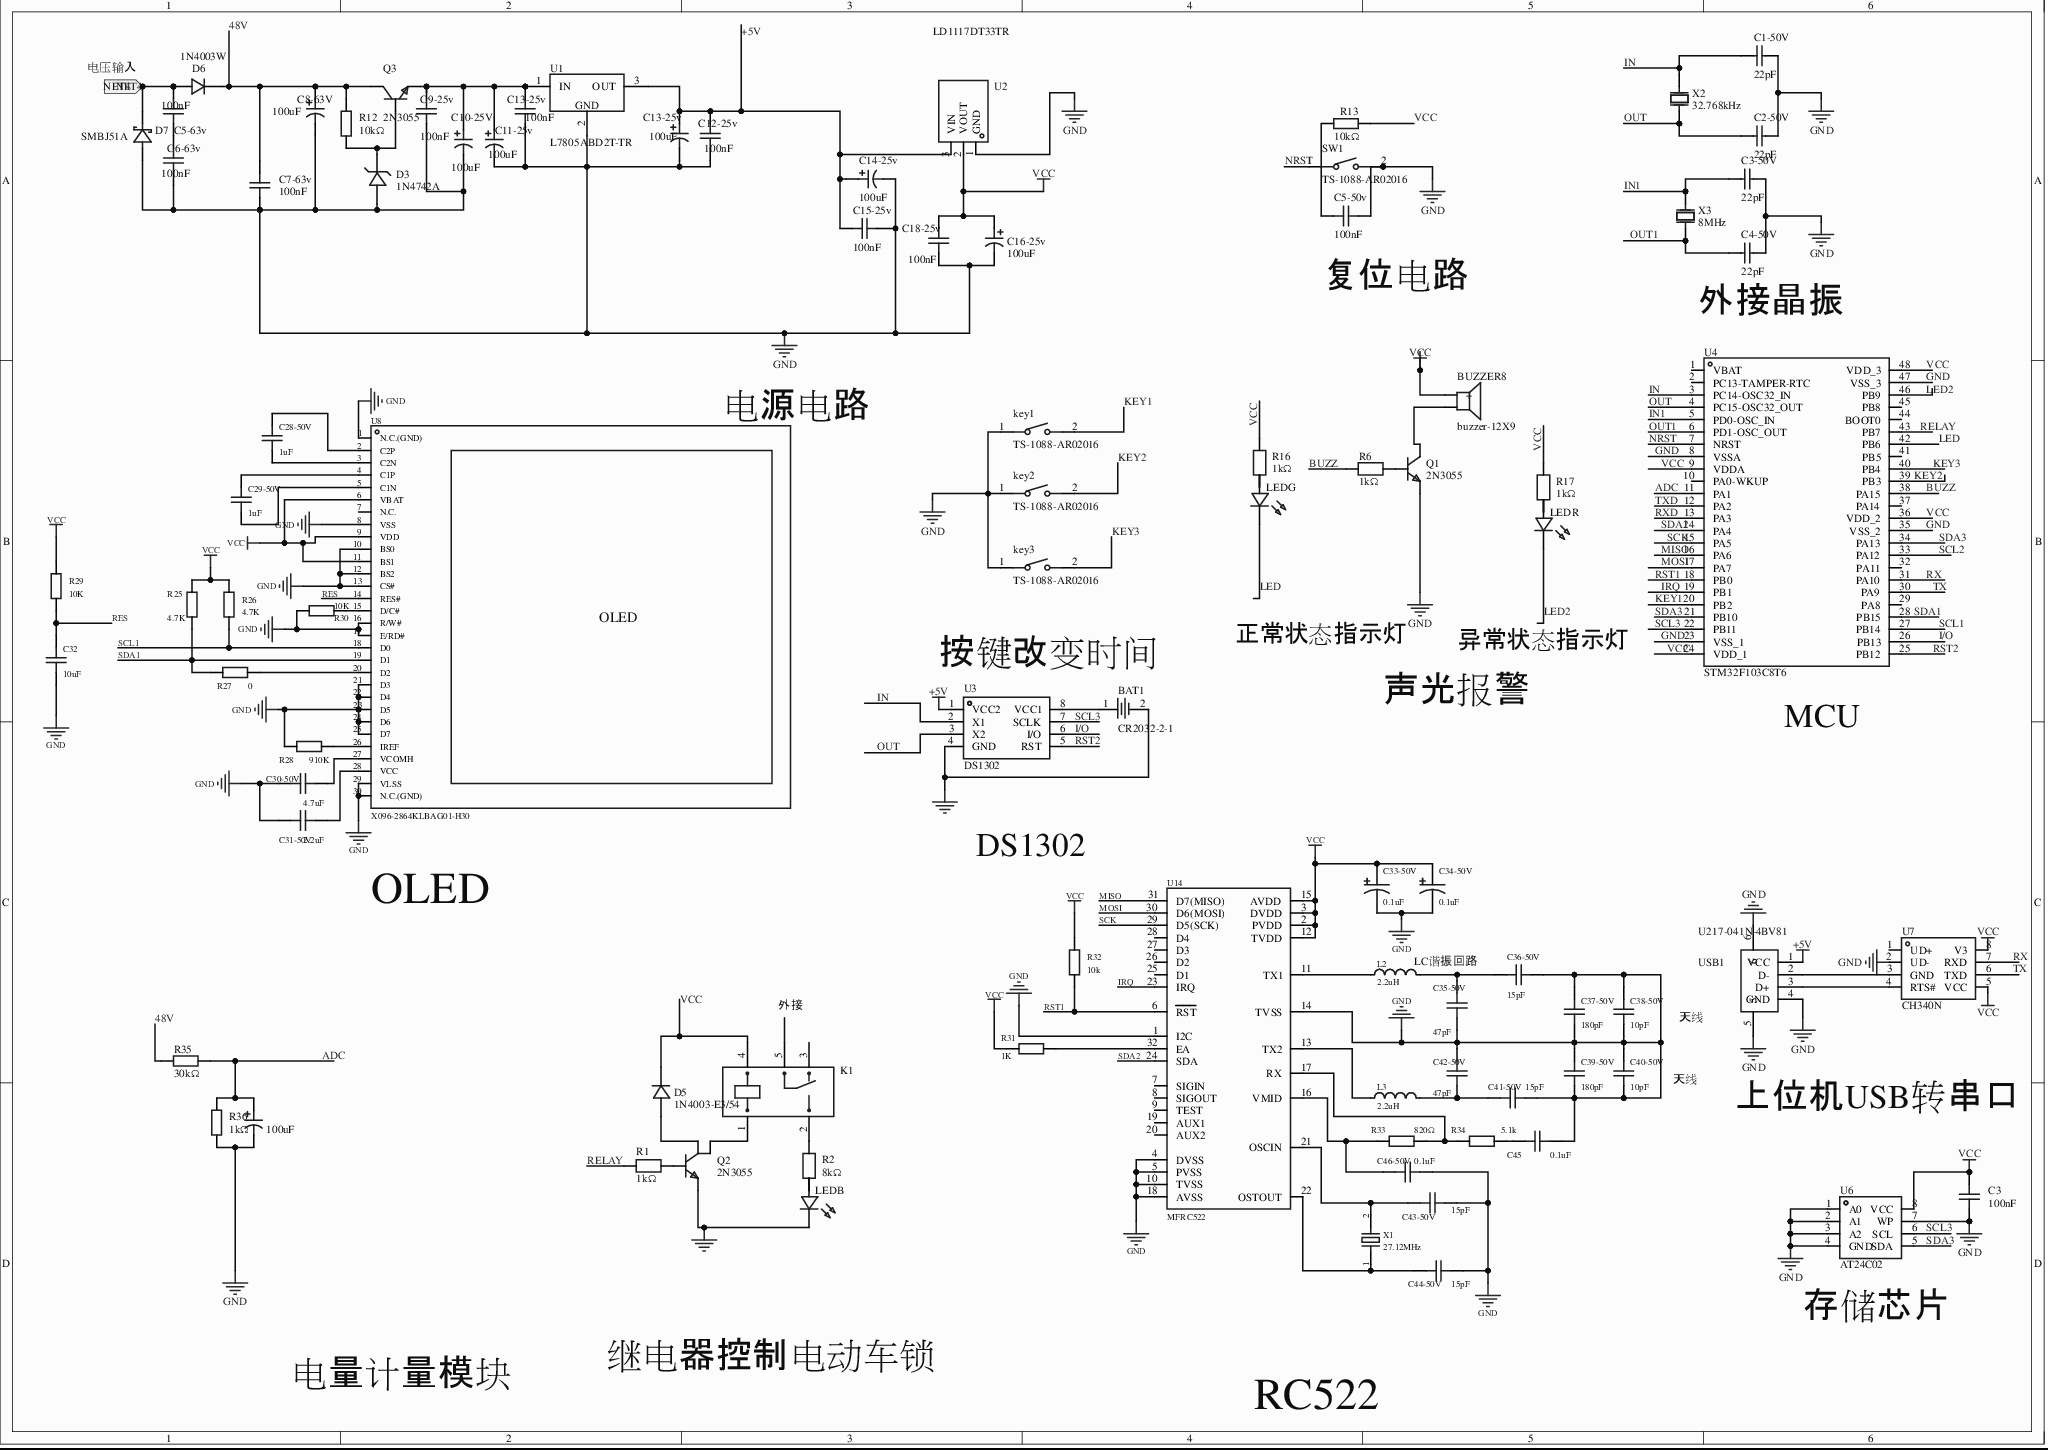
[diagram p0: MISC52145-3.schdoc]
# Altium project MISC52145-2.PrjPcb
1 sheet, 90 parts. Net scope: flat (ports and power ports of the same name join across sheets).
Board file: MISC52145.pcbdoc

## Sheet MISC52145-3.schdoc
size 420 x 297 mm; @Project Name: MISC52145; @Page Count: 1; @Update Date: 2026-04-09; @Create Date: 2026-04-09; @Schematic Name: MISC52145; @Page No: 1; @Board Name: MISC52145; @Create Time: 21:09:52; @Update Time: 10:26:27

### Parts
(Parts that share a designator on the sheet are numbered #1, #2 ... from top to bottom, then left to right.)
BAT1  CR2032-2-1  [BAT-TH_CR2032-2-1]
BUZZER8  buzzer-12X9  [BUZ-TH_BD12.0-P7.60-D0.6-FD]
C1-50V  22pF  [C0603]
C2-50V  22pF  [C0603]
C3  100nF  [C0603]
C3-50V  22pF  [C0603]
C4-50V  22pF  [C0603]
C5-50v  100nF  [C0603]
C5-63v#1  100nF  [C0603]
C5-63v#2  100uF  [CAP-SMD_BD10.0-L10.3-W10.3-LS11.0-FD_1]
C6-63v  100nF  [C0603]
C7-63v  100nF  [CAP-TH_L13.0-W6.0-P10.00-D1.0]
C8-63V  100uF  [CAP-SMD_BD6.3-L6.6-W6.6-LS7.3-FD-H7.7]
C9-25v  100nF  [CAP-TH_L13.0-W6.0-P10.00-D1.0]
C10-25V  100uF  [CAP-SMD_BD6.3-L6.6-W6.6-LS7.3-FD-H7.7]
C11-25v  100uF  [CAP-SMD_BD6.3-L6.6-W6.6-LS7.3-FD-H7.7]
C12-25v  100nF  [CAP-TH_L13.0-W6.0-P10.00-D1.0]
C13-25v#1  100nF  [CAP-TH_L13.0-W6.0-P10.00-D1.0]
C13-25v#2  100uF  [CAP-SMD_BD6.3-L6.6-W6.6-LS7.3-FD-H7.7]
C14-25v  100uF  [CAP-SMD_BD6.3-L6.6-W6.6-LS7.3-FD-H7.7]
C15-25v  100nF  [CAP-TH_L13.0-W6.0-P10.00-D1.0]
C16-25v  100uF  [CAP-SMD_BD6.3-L6.6-W6.6-LS7.3-FD-H7.7]
C18-25v  100nF  [CAP-TH_L13.0-W6.0-P10.00-D1.0]
C28-50V  1uF  [C0603]
C29-50V  1uF  [C0603]
C30-50V  4.7uF  [C0603]
C31-50V  2.2uF  [C0603]
C32  10uF  [C0603]
C33-50V  0.1uF  [CAP-SMD_BD5.0-L5.3-W5.3-FD]
C34-50V  0.1uF  [CAP-SMD_BD5.0-L5.3-W5.3-FD]
C35-50V  47pF  [C0603]
C36-50V  15pF  [C0603]
C37-50V  180pF  [C0603]
C38-50V  10pF  [C0603]
C39-50V  180pF  [C0603]
C40-50V  10pF  [C0603]
C41-50V  15pF  [C0603]
C42-50V  47pF  [C0603]
C43-50V  15pF  [C0603]
C44-50V  15pF  [C0603]
C45  0.1uF  [C0603]
C46-50V  0.1uF  [C0603]
D3  1N4742A  [DO-41_BD2.4-L4.7-P8.70-D0.9-RD]
D5  1N4003-E3/54  [DO-41_BD2.4-L4.7-P8.70-D0.9-RD]
D6  1N4003W  [SOD-123FL_L2.7-W1.8-LS3.8-RD]
D7  SMBJ51A  [SMB_L4.3-W3.6-LS5.4-R-RD]
K1  (no value)  [RELAY-TH_SRD-DCXXV-SL-C]
key1  TS-1088-AR02016  [SW-SMD_L3.9-W3.0-P4.45]
key2  TS-1088-AR02016  [SW-SMD_L3.9-W3.0-P4.45]
key3  TS-1088-AR02016  [SW-SMD_L3.9-W3.0-P4.45]
L2  2.2uH  [L0603]
L3  2.2uH  [L0603]
LEDB  (no value)  [LED_TH-3mm]
LEDG  (no value)  [LED_TH-3mm]
LEDR  (no value)  [LED_TH-3mm]
Q1  2N3055  [TO-3_L39.4-W26.7-P10.92-BL]
Q2  2N3055  [TO-3_L39.4-W26.7-P10.92-BL]
Q3  2N3055  [TO-3_L39.4-W26.7-P10.92-BL]
R1  value 1kΩ  [RES-TH_BD2.3-L6.5-P10.50-D0.5]
R2  value 8kΩ  [RES-TH_BD2.3-L6.5-P10.50-D0.5]
R6  value 1kΩ  [RES-TH_BD2.3-L6.5-P10.50-D0.5]
R12  10kΩ  [R0805]
R13  10kΩ  [R0805]
R16  value 1kΩ  [RES-TH_BD2.3-L6.5-P10.50-D0.5]
R17  value 1kΩ  [RES-TH_BD2.3-L6.5-P10.50-D0.5]
R25  4.7K  [R0603]
R26  4.7K  [R0603]
R27  0  [R0603]
R28  910K  [R0603]
R29  10K  [R0603]
R30  10K  [R0603]
R31  1K  [R0603]
R32  10k  [R0603]
R33  820Ω  [R0603]
R34  5.1k  [R0603]
R35  30kΩ  [R0603]
R36  1kΩ  [R0603]
SW1  TS-1088-AR02016  [SW-SMD_L3.9-W3.0-P4.45]
U1  L7805ABD2T-TR  [TO-263-2_L10.0-W9.2-P5.08-LS15.3-TL-CW]
U2  LD1117DT33TR  [TO-252-2_L6.6-W6.1-P4.57-LS9.9-BR-CW]
U3  DS1302  [DIP-8_L9.7-W6.4-P2.54-LS7.6-BL]
U4  STM32F103C8T6  [LQFP-48_L7.0-W7.0-P0.50-LS9.0-BL]
U5  MFRC522  [QFN32]  (value not drawn)
U6  AT24C02  [SOIC-8_L4.9-W3.9-P1.27-LS6.0-BL]
U7  CH340N  [SOP-8_L4.9-W3.9-P1.27-LS6.0-BL]
U8  X096-2864KLBAG01-H30  [OLED-SMD_X096-2864KLBAG01-H30]
USB1  U217-041N-4BV81  [USB-A-SMD_U217-041N-4BV81]
X1  27.12MHz  [OSC-SMD_L11.4-W4.5-LS12.5]
X2  32.768kHz  [CRYSTAL-SMD_L3.2-W1.5-1]
X3  8MHz  [CRYSTAL-SMD_L5.0-W3.2]

### Ports
NET4 (in)

### Nets
+5V: C12-25v.1 C13-25v#2.1 C14-25v.1 C15-25v.2 U1.3(OUT) U2.3(VIN) U3.1(VCC2) USB1.1(VCC)
GND: BAT1.2 BUZZER8.1(+) C1-50V.2 C2-50V.2 C3.1 C3.2 C3-50V.2 C4-50V.2 C5-50v.2 C5-63v#2.2 C6-63v.1 C7-63v.2 C8-63V.2 C9-25v.2 C10-25V.2 C11-25v.2 C12-25v.2 C13-25v#1.2 C13-25v#2.2 C14-25v.2 C15-25v.1 C16-25v.1 C16-25v.2 C18-25v.1 C18-25v.2 C30-50V.1 C31-50V.1 C32.1 C33-50V.1 C33-50V.2 C34-50V.1 C34-50V.2 C35-50V.1 C36-50V.2 C37-50V.1 C37-50V.2 C38-50V.1 C38-50V.2 C39-50V.1 C39-50V.2 C40-50V.1 C40-50V.2 C41-50V.2 C42-50V.2 C43-50V.1 C44-50V.1 C45.1 C46-50V.2 D3.2(A) D5.1(K) D7.1(A) K1.4 key1.1 key2.1 key3.1 LEDB.2(A) Q1.2(E) Q2.2(E) R13.1 R16.2 R17.2 R25.2 R26.2 R28.1 R29.2 R30.2 R31.1 R32.2 R36.1 SW1.2 U1.2(GND) U2.1(GND) U2.2(VOUT) U3.4(GND) U4.8(VSSA) U4.9(VDDA) U4.23(VSS_1) U4.24(VDD_1) U4.35(VSS_2) U4.36(VDD_2) U4.47(VSS_3) U4.48(VDD_3) U5.1(I2C) U5.2(PVDD) U5.3(DVDD) U5.4(DVSS) U5.5(PVSS) U5.10(TVSS) U5.12(TVDD) U5.14(TVSS) U5.15(AVDD) U5.18(AVSS) U6.1(A0) U6.2(A1) U6.3(A2) U6.4(GND) U6.7(WP) U6.8(VCC) U7.2(UD-) U7.5(VCC) U7.8(V3) U8.1(N.C.(GND)) U8.6(VBAT) U8.8(VSS) U8.9(VDD) U8.10(BS0) U8.11(BS1) U8.12(BS2) U8.13(CS#) U8.16(R/W#) U8.17(E/RD#) U8.21(D3) U8.22(D4) U8.23(D5) U8.24(D6) U8.25(D7) U8.29(VLSS) U8.30(N.C.(GND)) USB1.4(GND) USB1.5 USB1.6  [also labelled VCC]
48V: C7-63v.1 C8-63V.1 D6.1(K) Q3.3(C) R12.2 R35.1
ADC: C5-63v#2.1 R35.2 R36.2 U4.11(PA1)
BUZZ: R6.1 U4.38(PA15)
I/O: U3.6(I/O) U4.26(PB13)
IN: C1-50V.1 U3.2(X1) U4.3(PC14-OSC32_IN) X2.2(OSC2)
IN1: C3-50V.1 U4.5(PD0-OSC_IN) X3.2(OSC2)
IRQ: U4.19(PB1) U5.23(IRQ)
KEY1: key1.2 U4.20(PB2)
KEY2: key2.2 U4.39(PB3)
KEY3: key3.2 U4.40(PB4)
LED: LEDG.2(A) U4.42(PB6)
LED2: LEDR.2(A) U4.46(PB9)
MISO: U4.16(PA6) U5.31(D7(MISO))
MOSI: U4.17(PA7) U5.30(D6(MOSI))
NET4: C5-63v#1.2 D6.2(A) D7.2(K) ; port NET4
NRST: SW1.1 U4.7(NRST)
OUT: C2-50V.1 U3.3(X2) U4.4(PC15-OSC32_OUT) X2.1(OSC1)
OUT1: C4-50V.1 U4.6(PD1-OSC_OUT) X3.1(OSC1)
RELAY: R1.1 U4.43(PB7)
RES: C32.2 R29.1 U8.14(RES#)
RST1: R32.1 U4.18(PB0) U5.6(~{RST})
RST2: U3.5(RST) U4.25(PB12)
RX: U4.31(PA10) U7.7(RXD)
RXD: U4.13(PA3)
SCK: U4.15(PA5) U5.29(D5(SCK))
SCL1: R26.1 U4.27(PB14) U8.18(D0)
SCL2: U4.33(PA12)
SCL3: U3.7(SCLK) U4.22(PB11) U6.6(SCL)
SDA1: R25.1 R27.1 U4.28(PB15) U8.19(D1)
SDA2: U4.14(PA4) U5.24(SDA)
SDA3: U4.21(PB10) U4.34(PA13) U6.5(SDA)
TX: U4.30(PA9) U7.6(TXD)
TXD: U4.12(PA2)
NetBAT1_1: BAT1.1 U3.8(VCC1)
NetBUZZER8_2: BUZZER8.2 Q1.3(C)
NetC5-50v_1: C5-50v.1 R13.2
NetC5-63v#1_1: C5-63v#1.1 C6-63v.2
NetC9-25v_1: C9-25v.1 C10-25V.1 C11-25v.1 C13-25v#1.1 Q3.2(E) U1.1(IN)
NetC28-50V_1: C28-50V.1 U8.3(C2N)
NetC28-50V_2: C28-50V.2 U8.2(C2P)
NetC29-50V_1: C29-50V.1 U8.5(C1N)
NetC29-50V_2: C29-50V.2 U8.4(C1P)
NetC30-50V_2: C30-50V.2 U8.27(VCOMH)
NetC31-50V_2: C31-50V.2 U8.28(VCC)
NetC35-50V_2: C35-50V.2 C36-50V.1 L2.2
NetC41-50V_1: C41-50V.1 C42-50V.1 L3.2
NetC43-50V_2: C43-50V.2 U5.21(OSCIN) X1.2
NetC44-50V_2: C44-50V.2 U5.22(OSTOUT) X1.1
NetC45_2: C45.2 R34.2
NetC46-50V_1: C46-50V.1 R33.1 U5.16(VMID)
NetD3_1: D3.1(K) Q3.1(B) R12.1
NetD5_2: D5.2(A) Q2.3(C)
NetK1_1: K1.1 Q2.4(C)
NetK1_2: K1.2 R2.2
NetL2_1: L2.1 U5.11(TX1)
NetL3_1: L3.1 U5.13(TX2)
NetLEDB_1: LEDB.1(C) R2.1
NetLEDG_1: LEDG.1(C) R16.1
NetLEDR_1: LEDR.1(C) R17.1
NetQ1_1: Q1.1(B) R6.2
NetQ2_1: Q2.1(B) R1.2
NetR27_2: R27.2 U8.20(D2)
NetR28_2: R28.2 U8.26(IREF)
NetR30_1: R30.1 U8.15(D/C#)
NetR31_2: R31.2 U5.32(EA)
NetR33_2: R33.2 R34.1 U5.17(RX)
NetU7_3: U7.3(GND) USB1.2(D-)
NetU7_4: U7.4(RTS#) USB1.3(D+)

Not connected (* = marked no-connect by the designer): K1 3* 5; U4 1(VBAT)* 2(PC13-TAMPER-RTC)* 10(PA0-WKUP)* 29(PA8)* 32(PA11)* 37(PA14)* 41(PB5)* 44(BOOT0)* 45(PB8)*; U5 7(SIGIN)* 8(SIGOUT)* 9(TEST)* 19(AUX1)* 20(AUX2)* 25(D1)* 26(D2)* 27(D3)* 28(D4)*; U7 1(UD+)*; U8 7(N.C.)*

### Notes on the sheet
- 电压输入
- (near C5-50v) 复位电路
- 外接晶振
- 电源电路
- (near U3) 按键改变时间
- 正常状态指示灯
- 异常状态指示灯
- 声光报警
- (near U4) MCU
- OLED
- DS1302
- (near L2) LC谐振回路
- 外接
- 天线
- 上位机USB转串口
- (near U6) 存储芯片
- 电量计量模块
- 继电器控制电动车锁
- RC522

### Library data of the parts
BAT1 = CR2032-2-1: 3D Model: 9f297eb2328241df835384c32afd7d32; 3D Model Transform: 964.565,870.04,0,0,0,0,-42.047,0,-137.795; AddInBom: yes; Device: CR2032-2-1; Symbol: CR2032-2-1; LCSC Part Name: CR2032-2-1; Supplier Part: C9900018737; Manufacturer Part: CR2032-2-1; Supplier Footprint: BATTERY_CR2032-A; JLCPCB Part Class: 扩展库; Datasheet: https://atta.szlcsc.comnull; Supplier: LCSC; FootprintName: BAT-TH_CR2032-2-1; ConvertToPcb: yes; ModelName: BAT-TH_CR2032-2-1
BUZZER8 = buzzer-12X9: AddInBom: yes; ModelId: 16ab50e14c5b4f2c986c135bdba60e37; ModelName: BUZ-TH_D12.0-H9.5-P7.60; ModelTransform: 472.44,472.176,0,90,0,0,-0.787,0,-177.165; Device: buzzer-12X9; Symbol: buzzer-12X9; FootprintName: BUZ-TH_BD12.0-P7.60-D0.6-FD; LCSC Part Name: buzzer-12X9; SupplierPart: C9900016920; ManufacturerPart: buzzer-12X9; Supplier Footprint: BUZZER_SMT_9650B; JLCPCB Part Class: 扩展库; Datasheet: https://atta.szlcsc.comnull; Supplier: LCSC; ConvertToPcb: yes
C1-50V C2-50V C3-50V C4-50V = CL10C220JB8NNNC: 容值:22pF;精度:±5%;额定电压:50V;温度系数:C0G;; Manufacturer: SAMSUNG(三星); AddInBom: yes; Tolerance: ±5%; Voltage Rating: 50V; Temperature Coefficient: C0G; ModelId: ac125912035d415993ca9572d50418b10819f05c4eef4c71ace90d822a990e87; ModelName: C0603_L1.6-W0.8-H0.8; ModelTransform: 62.992,31.496,0,0,0,0,0,0,0; Device: CL10C220JB8NNNC; Symbol: CL10C220JB8NNNC; FootprintName: C0603; LCSC Part Name: 22pF ±5% 50V; SupplierPart: C1653; ManufacturerPart: CL10C220JB8NNNC; Supplier Footprint: 0603; JLCPCB Part Class: Basic Part; Datasheet: https://item.szlcsc.com/datasheet/CL10C220JB8NNNC/2005.html; Supplier: LCSC; ConvertToPcb: yes; Value: 22pF
C3 = CAP_0603: Symbol: Capacitance; ConvertToPcb: yes; ModelId: ac125912035d415993ca9572d50418b10819f05c4eef4c71ace90d822a990e87; ModelName: C0603_L1.6-W0.8-H0.8; ModelTransform: 62.992,31.496,0,0,0,0,0,0,0; Device: CAP_0603; FootprintName: C0603; AddInBom: yes; Supplier Footprint: 0603; Value: 100nF
C5-50v = CGA0603X7R104K500JT: 容值:100nF;精度:±10%;额定电压:50V;温度系数:X7R;; Manufacturer: HRE(芯声); AddInBom: yes; Tolerance: ±10%; Voltage Rating: 50V; Temperature Coefficient: X7R; ModelId: ac125912035d415993ca9572d50418b10819f05c4eef4c71ace90d822a990e87; ModelName: C0603_L1.6-W0.8-H0.8; ModelTransform: 62.992,31.496,0,0,0,0,0,0,0; Device: CGA0603X7R104K500JT; Symbol: CGA0603X7R104K500JT; FootprintName: C0603; LCSC Part Name: 100nF ±10% 50V; SupplierPart: C6119867; ManufacturerPart: CGA0603X7R104K500JT; Supplier Footprint: 0603; JLCPCB Part Class: Extended Part; Datasheet: https://item.szlcsc.com/datasheet/CGA0603X7R104K500JT/7062573.html; Supplier: LCSC; ConvertToPcb: yes; Value: 100nF
C5-63v#1 C6-63v = CGA0603X7R104K500JT: 容值:100nF;精度:±10%;额定电压:50V;温度系数:X7R;; Manufacturer: HRE(芯声); 3D Model: ac125912035d415993ca9572d50418b10819f05c4eef4c71ace90d822a990e87; 3D Model Transform: 62.992,31.496,0,0,0,0,0,0,0; Tolerance: ±10%; Voltage Rating: 50V; Temperature Coefficient: X7R; AddInBom: yes; ModelName: C0603_L1.6-W0.8-H0.8; Device: CGA0603X7R104K500JT; Symbol: CGA0603X7R104K500JT; LCSC Part Name: 100nF ±10% 50V; Supplier Part: C6119867; Manufacturer Part: CGA0603X7R104K500JT; Supplier Footprint: 0603; JLCPCB Part Class: Extended Part; Datasheet: https://item.szlcsc.com/datasheet/CGA0603X7R104K500JT/7062573.html; Supplier: LCSC; Value: 100nF; FootprintName: C0603; ConvertToPcb: yes
C5-63v#2 = RVT63V100M10X10: 容值:100uF;精度:±20%;额定电压:63V;纹波电流:200mA@120Hz;等效串联电阻(ESR):-;; Manufacturer: JIERR(捷而瑞); AddInBom: yes; Tolerance: ±20%; Voltage Rating: 63V; Lifetime: 2000hrs@105℃; Device: RVT63V100M10X10; Symbol: RVT63V100M10X10; FootprintName: CAP-SMD_BD10.0-L10.3-W10.3-LS11.0-FD_1; LCSC Part Name: 100uF ±20% 63V; SupplierPart: C51953411; ManufacturerPart: RVT63V100M10X10; Supplier Footprint: SMD,D10xL10.5mm; JLCPCB Part Class: Extended Part; Datasheet: https://item.szlcsc.com/datasheet/RVT63V100M10X10/54681536.html; Supplier: LCSC; ConvertToPcb: yes; Value: 100uF; Ripple Current: 200mA@120Hz; Equivalent Series Resistance(ESR): -; Diameter: 10mm; Height - Seated (Max): 10.5mm; Operating Temperature: -40℃~+105℃
C7-63v C9-25v C12-25v C13-25v#1 C15-25v C18-25v = MP2104K27C3X6LC: 容值:100nF;精度:±10%;工作电压(AC):275V;防护等级:X2;; Manufacturer: SRD(圣融达); Symbol: MP2104KGC3XLC; AddInBom: yes; Tolerance: ±10%; Voltage(AC): 275V; Ratings: X2; safety certification: UL；ENEC；VDE；CQC；CSA; ModelId: ab2ba9e918834f5e935e28a3e5a6a2b80819f05c4eef4c71ace90d822a990e87; ModelName: CAP-TH_L13.0-W6.0-H12.0-P10.0; ModelTransform: 511.81,236.22,0,0,0,0,0,0,-137.795; Device: MP2104K27C3X6LC; FootprintName: CAP-TH_L13.0-W6.0-P10.00-D1.0; LCSC Part Name: 100nF ±10% 275V 等级:X2; SupplierPart: C105759; ManufacturerPart: MP2104K27C3X6LC; Supplier Footprint: 插件,P=10mm; JLCPCB Part Class: Extended Part; Datasheet: https://item.szlcsc.com/datasheet/MP2104K27C3X6LC/106974.html; Supplier: LCSC; ConvertToPcb: yes; Value: 100nF
C8-63V C14-25v C16-25v = JVJ50V100M6x8: 容值:100uF;精度:±20%;额定电压:50V;纹波电流:140mA@120Hz;; Manufacturer: JIERR(捷而瑞); 3D Model: ccbda52dceed4b139172c40f75c9da3f0819f05c4eef4c71ace90d822a990e87; 3D Model Transform: 287.401,259.842,0,0,0,0,0,0,0; Tolerance: ±20%; Voltage Rating: 50V; Lifetime: 2000hrs@105℃; AddInBom: yes; Device: JVJ50V100M6x8; Symbol: JVJ50V100M6X8; LCSC Part Name: 100uF ±20% 50V; Supplier Part: C46550415; Manufacturer Part: JVJ50V100M6x8; Supplier Footprint: SMD,D6.3xL7.7mm; JLCPCB Part Class: Extended Part; Datasheet: https://item.szlcsc.com/datasheet/JVJ50V100M6x8/48680109.html; Supplier: LCSC; Value: 100uF; Ripple Current: 140mA@120Hz; Diameter: 6.3mm; Height - Seated (Max): 7.7mm; Operating Temperature: -55℃~+105℃; FootprintName: CAP-SMD_BD6.3-L6.6-W6.6-LS7.3-FD-H7.7; ConvertToPcb: yes; ModelName: CAP-SMD_BD6.3-L6.6-W6.6-LS7.3-FD-H7.7
C10-25V C11-25v C13-25v#2 = JVJ50V100M6x8: 容值:100uF;精度:±20%;额定电压:50V;纹波电流:140mA@120Hz;; Manufacturer: JIERR(捷而瑞); AddInBom: yes; Tolerance: ±20%; Voltage Rating: 50V; Lifetime: 2000hrs@105℃; ModelId: ccbda52dceed4b139172c40f75c9da3f0819f05c4eef4c71ace90d822a990e87; ModelTransform: 287.401,259.842,0,0,0,0,0,0,0; Device: JVJ50V100M6x8; Symbol: JVJ50V100M6X8; FootprintName: CAP-SMD_BD6.3-L6.6-W6.6-LS7.3-FD-H7.7; LCSC Part Name: 100uF ±20% 50V; SupplierPart: C46550415; ManufacturerPart: JVJ50V100M6x8; Supplier Footprint: SMD,D6.3xL7.7mm; JLCPCB Part Class: Extended Part; Datasheet: https://item.szlcsc.com/datasheet/JVJ50V100M6x8/48680109.html; Supplier: LCSC; ConvertToPcb: yes; Value: 100uF; Ripple Current: 140mA@120Hz; Diameter: 6.3mm; Height - Seated (Max): 7.7mm; Operating Temperature: -55℃~+105℃; ModelName: CAP-SMD_BD6.3-L6.6-W6.6-LS7.3-FD-H7.7
C28-50V C29-50V C30-50V C31-50V C32 C35-50V C36-50V C37-50V C38-50V C39-50V C40-50V C41-50V C42-50V C43-50V C44-50V C45 C46-50V = CAP_0603: Symbol: Capacitance; 3D Model: ac125912035d415993ca9572d50418b10819f05c4eef4c71ace90d822a990e87; 3D Model Transform: 62.992,31.496,0,0,0,0,0,0,0; ConvertToPcb: yes; ModelName: C0603_L1.6-W0.8-H0.8; Device: CAP_0603; Supplier Footprint: 0603; FootprintName: C0603; AddInBom: yes
  C28-50V C29-50V: Value: 1uF
  C30-50V: Value: 4.7uF
  C31-50V: Value: 2.2uF
  C32: Value: 10uF
  C35-50V C42-50V: Value: 47pF
  C36-50V C41-50V C43-50V C44-50V: Value: 15pF
  C37-50V C39-50V: Value: 180pF
  C38-50V C40-50V: Value: 10pF
  C45 C46-50V: Value: 0.1uF
C33-50V C34-50V = EMVE500ADA4R7ME55G: 容值:4.7uF;精度:±20%;额定电压:50V;纹波电流:20mA@120Hz;等效串联电阻(ESR):-;; Manufacturer: NCC(日本贵弥功); 3D Model: 16f5696d655347d6a4362817d02ce59a0819f05c4eef4c71ace90d822a990e87; 3D Model Transform: 216.535,208.661,0,0,0,0,0,0,0; Tolerance: ±20%; Voltage Rating: 50V; Lifetime: 1000hrs@105℃; AddInBom: yes; ModelName: CAP-SMD_BD5.0-L5.3-W5.3-LS5.5-FD; Device: EMVE500ADA4R7ME55G; Symbol: EMVE500ADA4R7ME55G; Value: 0.1uF; LCSC Part Name: 4.7uF ±20% 50V; Manufacturer Part: EMVE500ADA4R7ME55G; Supplier Footprint: SMD,D5xL5.2mm; JLCPCB Part Class: Extended Part; Datasheet: https://item.szlcsc.com/datasheet/EMVE500ADA4R7ME55G/189663.html; Supplier: LCSC; Ripple Current: 20mA@120Hz; Equivalent Series Resistance(ESR): -; Diameter: 5mm; Height - Seated (Max): 5.2mm; Operating Temperature: -40℃~+105℃; FootprintName: CAP-SMD_BD5.0-L5.3-W5.3-FD; ConvertToPcb: yes
D3 = 1N4742A_C140853: 二极管配置:独立式;稳压值(标称值):12V;稳压值(范围):11.4V~12.6V;耗散功率(Pd):1W;; Manufacturer: onsemi(安森美); AddInBom: yes; Diode Configuration: 独立式; Zener Voltage(Nom): 12V; Reverse Leakage Current (Ir): 5uA@9.1V; Pd - Power Dissipation: 1W; Impedance(Zzt): 9Ω; Impedance(Zzk): 700Ω; Operating Junction Temperature Range: -65℃~+200℃; ModelId: 6de1e9b71a0d4751b4e9df530304c1a30819f05c4eef4c71ace90d822a990e87; ModelName: DO-41_D2.4-L4.7-P8.70; ModelTransform: 374.016,94.488,0,0,0,0,0,0,-137.795; Device: 1N4742A_C140853; Symbol: 1N4742A_C140853; FootprintName: DO-41_BD2.4-L4.7-P8.70-D0.9-RD; LCSC Part Name: 独立式 耐压:12V 电流:5uA@9.1V; SupplierPart: C140853; ManufacturerPart: 1N4742A; Supplier Footprint: DO-41; JLCPCB Part Class: Extended Part; Datasheet: https://item.szlcsc.com/datasheet/1N4742A/152181.html; Supplier: LCSC; ConvertToPcb: yes; Zener Voltage(Range): 11.4V~12.6V
D5 = 1N4003-E3/54: 二极管配置:-;正向压降(Vf):1.1V@1A;直流反向耐压(Vr):200V;整流电流:1A;; Manufacturer: VISHAY(威世); AddInBom: yes; Voltage - DC Reverse(Vr): 200V; Current - Rectified: 1A; Reverse Leakage Current (Ir): 5uA@200V; Non-Repetitive Peak Forward Surge Current: 45A; Operating Junction Temperature Range: -50℃~+150℃; ModelId: 6de1e9b71a0d4751b4e9df530304c1a30819f05c4eef4c71ace90d822a990e87; ModelName: DO-41_D2.4-L4.7-P8.70; ModelTransform: 374.016,94.488,0,0,0,0,0,0,-137.795; Device: 1N4003-E3/54; Symbol: 1N4003-E3/54; FootprintName: DO-41_BD2.4-L4.7-P8.70-D0.9-RD; LCSC Part Name: 通用型塑封整流器; SupplierPart: C143068; ManufacturerPart: 1N4003-E3/54; Supplier Footprint: DO-41; JLCPCB Part Class: Extended Part; Datasheet: https://item.szlcsc.com/datasheet/1N4003-E3%252F54/154399.html; Supplier: LCSC; ConvertToPcb: yes; Diode Configuration: -; Voltage - Forward(Vf@If): 1.1V@1A
D6 = 1N4003W: 二极管配置:独立式;正向压降(Vf):1.1V@1A;直流反向耐压(Vr):200V;整流电流:1A;; Manufacturer: 晶导微电子; AddInBom: yes; Diode Configuration: 独立式; Voltage - DC Reverse(Vr): 200V; Current - Rectified: 1A; Reverse Leakage Current (Ir): 5uA@200V; ModelId: 86f9151e155e4fe2af0c4f2e0a80302e0819f05c4eef4c71ace90d822a990e87; ModelName: SOD-123FL_L2.8-W1.8-H1.1-LS3.6; ModelTransform: 141.732,70.866,0,180,0,0,0,0,0; Device: 1N4003W; Symbol: 1N4003W; FootprintName: SOD-123FL_L2.7-W1.8-LS3.8-RD; LCSC Part Name: 200V 1A; SupplierPart: C437592; ManufacturerPart: 1N4003W; Supplier Footprint: SOD-123FL; JLCPCB Part Class: Extended Part; Datasheet: https://item.szlcsc.com/datasheet/1N4003W/436156.html; Supplier: LCSC; ConvertToPcb: yes; Voltage - Forward(Vf@If): 1.1V@1A
D7 = SMBJ51A_C1973217: 极性:单向;反向截止电压(Vrwm):51V;钳位电压:82.4V;峰值脉冲电流(Ipp):7.3A@10/1000us;峰值脉冲功率(Ppp):600W@10/1000us;击穿电压:62.7V;; Manufacturer: Littelfuse(美国力特); AddInBom: yes; Polarity: 单向; Reverse Stand-Off Voltage (Vrwm): 51V; Clamping Voltage: 82.4V; Voltage - Breakdown: 62.7V; Reverse Leakage Current (Ir): 1uA; level of protection: IEC 61000-4-4；IEC 61000-4-2; Type: TVS; ModelId: 89ecc9465fc8412eb5ba544f68f54b7c0819f05c4eef4c71ace90d822a990e87; ModelTransform: 214.1728,140.1572,0,0,0,0,0,0,0; Device: SMBJ51A_C1973217; Symbol: SMBJ51A_C1973217; FootprintName: SMB_L4.3-W3.6-LS5.4-R-RD; LCSC Part Name: 单向TVS 51V截止 峰值脉冲电流：7.3A@10/1000us; SupplierPart: C1973217; ManufacturerPart: SMBJ51A; Supplier Footprint: DO-214AA; JLCPCB Part Class: Extended Part; Datasheet: https://item.szlcsc.com/datasheet/SMBJ51A/2064755.html; Supplier: LCSC; ConvertToPcb: yes; Peak Pulse Current (Ipp): 7.3A@10/1000us; Peak Pulse Power Dissipation (Ppp): 600W@10/1000us; Operating Temperature: -65℃~+150℃; ModelName: SMB_L4.3-W3.6-LS5.4-R-RD
K1 = SRD-DC5V-SL-C: 继电器类型:-;线圈类型:-;线圈电压:-;触点形式:-;触点的额定电流:-;; 3D Model: 599951857ec9401b9cd71ea2bb1edaba; 3D Model Transform: 755.9,779.5,0,0,90,0,35.4,307.1,248; AddInBom: yes; ModelName: RELAY-TH_L19.2-W15.6-H15.8; Device: SRD-DC5V-SL-C; Symbol: SRD-DC5V-SL-C; LCSC Part Name: SRD-DC5V-SL-C; Supplier Part: C688865; Manufacturer Part: SRD-DC5V-SL-C; Supplier Footprint: 插件; JLCPCB Part Class: 扩展库; Datasheet: https://atta.szlcsc.com/upload/public/pdf/source/20200305/C490149_C96E4098A3B1FFB377D5AD2E40B7C2A8.pdf; Supplier: LCSC; Relay Type: -; Coil Type: -; Coil Voltage: -; Contact Form: -; Contact Rating (Current): -; Switching Voltage: -; FootprintName: RELAY-TH_SRD-DCXXV-SL-C; ConvertToPcb: yes
key1-key3 SW1 = TS-1088-AR02016: 电路结构:单刀单掷;按钮形状:圆形按钮;作用力:1.6N;安装方式:立贴;开关长度:4mm;开关宽度:3mm;开关高度:2mm;带支架:不带支架;触点电流:50mA;额定电压:12V;工作寿命:10万次;; Manufacturer: XUNPU(讯普); AddInBom: yes; Circuit: 单刀单掷; Actuator Style: 圆形按钮; Operating Force: 1.6N; Switch Height: 2mm; with Bracket: 不带支架; Contact Current: 50mA; Voltage Rating: 12V; Actuator/Cap Color: 黑色; Life: 10万次; ModelId: b26698b69f274ffabef8a26c7d0e5dd10819f05c4eef4c71ace90d822a990e87; ModelName: SW-SMD_L3.9-W2.9-H2.0-LS4.8; ModelTransform: 188.976,114.174,0,0,0,0,0,0,0; Device: TS-1088-AR02016; Symbol: TS-1088-AR02016; FootprintName: SW-SMD_L3.9-W3.0-P4.45; LCSC Part Name: 4*3*2mm 立贴 轻触开关; SupplierPart: C720477; ManufacturerPart: TS-1088-AR02016; Supplier Footprint: SMD,4x3mm; JLCPCB Part Class: Basic Part; Datasheet: https://item.szlcsc.com/datasheet/TS-1088-AR02016/763484.html; Supplier: LCSC; ConvertToPcb: yes; Mounting Type: 立贴; Length: 4mm; Width: 3mm; Termination Style: SMD接片; Operating Temperature: -30℃~+80℃
L2 L3 = L_0603: Symbol: SDFL1608S100KTF; 3D Model: 2bc5ec593d464d6ba9807aec0b5673c20819f05c4eef4c71ace90d822a990e87; 3D Model Transform: 62.992,31.496,0,180,0,0,0.094,0.629,0; AddInBom: yes; ModelName: L0603_L1.6-W0.8-H0.5_BEAD; Device: L_0603; Supplier Footprint: L0603; Value: 2.2uH; FootprintName: L0603; ConvertToPcb: yes
LEDB LEDG LEDR = LED_TH-B_3mm: 3D Model: ff771fff7070432ca3f353cf0f67af4c0819f05c4eef4c71ace90d822a990e87; 3D Model Transform: 134.36,149.37,405.47,0,0,0,-11.81,0,-196.85; ConvertToPcb: yes; ModelName: LED-TH_BD3.8-P2.54-FD_BLUE; Device: LED_TH-B_3mm; Symbol: LED_TH-B; Supplier Footprint: 插件; FootprintName: LED_TH-3mm; AddInBom: yes
Q1 = 2N3055_C2848354: 晶体管类型:NPN;集电极电流(Ic):15A;集射极击穿电压(Vceo):60V;耗散功率(Pd):115W;直流电流增益(hFE):5@10A,4V;; Manufacturer: JSMSEMI(杰盛微); Symbol: 2N3055_C2848354_1; type: NPN; Current - Collector(Ic): 15A; Collector - Emitter Voltage VCEO: 60V; Pd - Power Dissipation: 115W; Transition frequency(fT): 2.5MHz; Current - Collector Cutoff: 700uA; Vce Saturation(VCE(sat)): 3V@10A,3.3A; Emitter-Base Voltage(Vebo): 7V; 3D Model: f20eabb5ebdf4a27883e614f62697bb60819f05c4eef4c71ace90d822a990e87; 3D Model Transform: 1048.982,1549.99682,0,0,0,0,0,0,-472.441; AddInBom: yes; ModelName: TO-3_L39.4-W26.7-H8.5-P10.92-BL; Device: 2N3055_C2848354; LCSC Part Name: NPN 电流:15A 电压:60V; Supplier Part: C2848354; Manufacturer Part: 2N3055; Supplier Footprint: TO-3; JLCPCB Part Class: Extended Part; Datasheet: https://item.szlcsc.com/datasheet/2N3055/3047496.html; Supplier: LCSC; DC Current Gain: 5@10A,4V; Operating Temperature: -65℃~+150℃@(Tj); FootprintName: TO-3_L39.4-W26.7-P10.92-BL; ConvertToPcb: yes
Q2 = 2N3055_C2848354: 晶体管类型:NPN;集电极电流(Ic):15A;集射极击穿电压(Vceo):60V;耗散功率(Pd):115W;直流电流增益(hFE):5@10A,4V;; Manufacturer: JSMSEMI(杰盛微); AddInBom: yes; type: NPN; Current - Collector(Ic): 15A; Collector - Emitter Voltage VCEO: 60V; Pd - Power Dissipation: 115W; Transition frequency(fT): 2.5MHz; Current - Collector Cutoff: 700uA; Vce Saturation(VCE(sat)): 3V@10A,3.3A; Emitter-Base Voltage(Vebo): 7V; ModelId: f20eabb5ebdf4a27883e614f62697bb60819f05c4eef4c71ace90d822a990e87; ModelName: TO-3_L39.4-W26.7-H8.5-P10.92-BL; ModelTransform: 1048.982,1549.99682,0,0,0,0,0,0,-472.441; Device: 2N3055_C2848354; Symbol: 2N3055_C2848354; FootprintName: TO-3_L39.4-W26.7-P10.92-BL; LCSC Part Name: NPN 电流:15A 电压:60V; SupplierPart: C2848354; ManufacturerPart: 2N3055; Supplier Footprint: TO-3; JLCPCB Part Class: Extended Part; Datasheet: https://item.szlcsc.com/datasheet/2N3055/3047496.html; Supplier: LCSC; ConvertToPcb: yes; DC Current Gain: 5@10A,4V; Operating Temperature: -65℃~+150℃@(Tj)
Q3 = 2N3055_C2848354: 晶体管类型:NPN;集电极电流(Ic):15A;集射极击穿电压(Vceo):60V;耗散功率(Pd):115W;直流电流增益(hFE):5@10A,4V;; Manufacturer: JSMSEMI(杰盛微); Symbol: 2N3055_C2848354_1; AddInBom: yes; type: NPN; Current - Collector(Ic): 15A; Collector - Emitter Voltage VCEO: 60V; Pd - Power Dissipation: 115W; Transition frequency(fT): 2.5MHz; Current - Collector Cutoff: 700uA; Vce Saturation(VCE(sat)): 3V@10A,3.3A; Emitter-Base Voltage(Vebo): 7V; ModelId: f20eabb5ebdf4a27883e614f62697bb60819f05c4eef4c71ace90d822a990e87; ModelName: TO-3_L39.4-W26.7-H8.5-P10.92-BL; ModelTransform: 1048.982,1549.99682,0,0,0,0,0,0,-472.441; Device: 2N3055_C2848354; FootprintName: TO-3_L39.4-W26.7-P10.92-BL; LCSC Part Name: NPN 电流:15A 电压:60V; SupplierPart: C2848354; ManufacturerPart: 2N3055; Supplier Footprint: TO-3; JLCPCB Part Class: Extended Part; Datasheet: https://item.szlcsc.com/datasheet/2N3055/3047496.html; Supplier: LCSC; ConvertToPcb: yes; DC Current Gain: 5@10A,4V; Operating Temperature: -65℃~+150℃@(Tj)
R1 R2 R16 R17 = 插件电阻: 电阻类型:金属膜电阻;阻值:1kΩ;精度:±1%;功率:500mWS;温度系数:±50ppm/℃;工作温度范围:-;; Manufacturer: Tyohm(幸亚电阻); Symbol: RN1/2WS1KΩFT/BA1; 3D Model: 8e6c7ee8323443d1ab8f0504b6353c8c; 3D Model Transform: 431.1015,91.3384,0,0,0,0,0.197,0,-137.795; Tolerance: ±1%; Power(Watts): 500mWS; AddInBom: yes; ModelName: RES-TH_D2.3-L6.5-P10.50; Device: 插件电阻; LCSC Part Name: 1kΩ ±1% 500mWS; Manufacturer Part: RN1/2WS1KΩFT/BA1; Supplier Footprint: 轴向引线; JLCPCB Part Class: 扩展库; Datasheet: https://atta.szlcsc.com/upload/public/pdf/source/20190522/C385463_1A74B5322676C5D38AC622BB88C12821.pdf; Supplier: LCSC; Type: 金属膜电阻; Temperature Coefficient: ±50ppm/℃; Operating Temperature Range: -; FootprintName: RES-TH_BD2.3-L6.5-P10.50-D0.5; ConvertToPcb: yes
  R1 R16 R17: Supplier Part: C385463
R6 = 插件电阻: 电阻类型:金属膜电阻;阻值:1kΩ;精度:±1%;功率:500mWS;温度系数:±50ppm/℃;工作温度范围:-;; Manufacturer: Tyohm(幸亚电阻); Symbol: RN1/2WS1KΩFT/BA1; AddInBom: yes; Tolerance: ±1%; Power(Watts): 500mWS; ModelId: 8e6c7ee8323443d1ab8f0504b6353c8c; ModelName: RES-TH_D2.3-L6.5-P10.50; ModelTransform: 431.1015,91.3384,0,0,0,0,0.197,0,-137.795; Device: 插件电阻; FootprintName: RES-TH_BD2.3-L6.5-P10.50-D0.5; LCSC Part Name: 1kΩ ±1% 500mWS; SupplierPart: C385463; ManufacturerPart: RN1/2WS1KΩFT/BA1; Supplier Footprint: 轴向引线; JLCPCB Part Class: 扩展库; Datasheet: https://atta.szlcsc.com/upload/public/pdf/source/20190522/C385463_1A74B5322676C5D38AC622BB88C12821.pdf; Supplier: LCSC; ConvertToPcb: yes; Type: 金属膜电阻; Temperature Coefficient: ±50ppm/℃; Operating Temperature Range: -
R12 R13 = 0805W8F1002T5E_C17414: 电阻类型:厚膜电阻;阻值:10kΩ;精度:±1%;功率:125mW;工作电压:150V;温度系数:±100ppm/℃;; Manufacturer: UNI-ROYAL(厚声); AddInBom: yes; Tolerance: ±1%; Power(Watts): 125mW; Voltage-Supply(Max): 150V; ModelId: 37a81e68749a4138bd2dfa6897b24b850819f05c4eef4c71ace90d822a990e87; ModelName: R0805_L2.0-W1.3-H0.6; ModelTransform: 78.74,51.181,0,0,0,0,0,-0.0005,0; Device: 0805W8F1002T5E_C17414; Symbol: 0805W8F1002T5E; FootprintName: R0805; LCSC Part Name: 10kΩ ±1% 125mW 厚膜电阻; SupplierPart: C17414; ManufacturerPart: 0805W8F1002T5E; Supplier Footprint: 0805; JLCPCB Part Class: Basic Part; Datasheet: https://item.szlcsc.com/datasheet/0805W8F1002T5E/18102.html; Supplier: LCSC; ConvertToPcb: yes; Type: 厚膜电阻; Value: 10kΩ; Temperature Coefficient: ±100ppm/℃; Operating Temperature: -55℃~+155℃
R25-R34 = Res_0603: Symbol: 电阻; 3D Model: fc143cca1e79419f9cd78b61e9279f080819f05c4eef4c71ace90d822a990e87; 3D Model Transform: 31.8897,63.7794,0,90,0,0,0,0,0; ConvertToPcb: yes; Device: Res_0603; Supplier Footprint: 0603; FootprintName: R0603; AddInBom: yes; ModelName: R0603
  R25 R26: Value: 4.7K
  R27: Value: 0
  R28: Value: 910K
  R29 R30: Value: 10K
  R31: Value: 1K
  R32: Value: 10k
  R33: Value: 820Ω
  R34: Value: 5.1k
R35 = 0603WAF3002T5E: 电阻类型:厚膜电阻;阻值:30kΩ;精度:±1%;功率:100mW;工作电压:75V;温度系数:±100ppm/℃;; Manufacturer: UNI-ROYAL(厚声); AddInBom: yes; Tolerance: ±1%; Power(Watts): 100mW; Voltage-Supply(Max): 75V; ModelId: fc143cca1e79419f9cd78b61e9279f080819f05c4eef4c71ace90d822a990e87; ModelTransform: 31.8897,63.7794,0,90,0,0,0,0,0; Device: 0603WAF3002T5E; Symbol: 0603WAF3002T5E; FootprintName: R0603; LCSC Part Name: 30kΩ ±1% 100mW 厚膜电阻; SupplierPart: C22984; ManufacturerPart: 0603WAF3002T5E; Supplier Footprint: 0603; JLCPCB Part Class: Basic Part; Datasheet: https://item.szlcsc.com/datasheet/0603WAF3002T5E/23711.html; Supplier: LCSC; ConvertToPcb: yes; Type: 厚膜电阻; Value: 30kΩ; Temperature Coefficient: ±100ppm/℃; Operating Temperature: -55℃~+155℃; ModelName: R0603
R36 = 0603WAF1001T5E: 电阻类型:厚膜电阻;阻值:1kΩ;精度:±1%;功率:100mW;工作电压:75V;温度系数:±100ppm/℃;; Manufacturer: UNI-ROYAL(厚声); 3D Model: fc143cca1e79419f9cd78b61e9279f080819f05c4eef4c71ace90d822a990e87; 3D Model Transform: 31.8897,63.7794,0,90,0,0,0,0,0; Tolerance: ±1%; Power(Watts): 100mW; Voltage-Supply(Max): 75V; AddInBom: yes; Device: 0603WAF1001T5E; Symbol: 0603WAF1001T5E; LCSC Part Name: 1kΩ ±1% 100mW 厚膜电阻; Supplier Part: C21190; Manufacturer Part: 0603WAF1001T5E; Supplier Footprint: 0603; JLCPCB Part Class: Basic Part; Datasheet: https://item.szlcsc.com/datasheet/0603WAF1001T5E/21904.html; Supplier: LCSC; Type: 厚膜电阻; Value: 1kΩ; Temperature Coefficient: ±100ppm/℃; Operating Temperature: -55℃~+155℃; FootprintName: R0603; ConvertToPcb: yes; ModelName: R0603
U1 = L7805ABD2T-TR: 输出类型:固定;工作电压:35V;输出电压:5V;输出电流:1.5A;电源纹波抑制比(PSRR):68dB@(120Hz);输出极性:正极;; Manufacturer: ST(意法半导体); AddInBom: yes; Output Type: 固定; Voltage - Supply: 35V; Output Voltage: 5V; Output Current: 1.5A; Voltage Dropout: 2V@(1A); standby current: 4.3mA; Output Configuration: 正极; Number of Outputs: 1; ModelId: d0164c4729fb485ab05f312a49c96c520819f05c4eef4c71ace90d822a990e87; ModelName: TO-263-2_L10.2-W8.7-H4.5-LS15.2-P2.54; ModelTransform: 401.574,591.64307,0,270,0,0,54.134,0.079,0; Device: L7805ABD2T-TR; Symbol: L7805ABD2T-TR; FootprintName: TO-263-2_L10.0-W9.2-P5.08-LS15.3-TL-CW; LCSC Part Name: 正稳压器IC; SupplierPart: C86206; ManufacturerPart: L7805ABD2T-TR; Supplier Footprint: TO-263-2; JLCPCB Part Class: Extended Part; Datasheet: https://item.szlcsc.com/datasheet/L7805ABD2T-TR/87382.html; Supplier: LCSC; ConvertToPcb: yes; Power Supply Rejection Ratio (PSRR): 68dB@(120Hz); Noise: -; Features: 短路保护；过热保护; Operating Temperature: -40℃~+125℃@(Tj)
U2 = LD1117DT33TR: 输出类型:固定;工作电压:15V;输出电压:3.3V;输出电流:800mA;电源纹波抑制比(PSRR):75dB@(120Hz);输出极性:正极;; Manufacturer: ST(意法半导体); AddInBom: yes; Output Type: 固定; Voltage - Supply: 15V; Output Voltage: 3.3V; Output Current: 800mA; Voltage Dropout: 1.2V@(800mA); standby current: 5mA; Noise: 100uVrms; Output Configuration: 正极; Number of Outputs: 1; ModelId: ce57f84d66384067af8a68020b6de06d0819f05c4eef4c71ace90d822a990e87; ModelName: TO-252-2L-3P_L6.6-W6.1-H2.3-LS10.1-P4.6; ModelTransform: 259.842,390.52442,0,90,0,0,-39.39,0,0; Device: LD1117DT33TR; Symbol: LD1117DT33TR; FootprintName: TO-252-2_L6.6-W6.1-P4.57-LS9.9-BR-CW; LCSC Part Name: 3.3V 800mA 15V; SupplierPart: C132629; ManufacturerPart: LD1117DT33TR; Supplier Footprint: TO-252-2; JLCPCB Part Class: Extended Part; Datasheet: https://item.szlcsc.com/datasheet/LD1117DT33TR/143929.html; Supplier: LCSC; ConvertToPcb: yes; Power Supply Rejection Ratio (PSRR): 75dB@(120Hz); Features: 过热保护；过流保护; Operating Temperature: 0℃~+125℃@(Tj)
U3 = DS1302N: Manufacturer: HGSEMI(华冠); 3D Model: 5746b540d01a4d1b9eb6b4f989297bc7; 3D Model Transform: 385.826,311.8104,0,0,0,0,0,0,-118.11; AddInBom: yes; ModelName: DIP-8_L9.8-W6.6-H3.5-LS7.62-P2.54; Device: DS1302N; Symbol: DS1302N; Manufacturer Part: DS1302; LCSC Part Name: DS1302N; Supplier Part: C398065; Supplier Footprint: DIP-8; JLCPCB Part Class: 扩展库; Datasheet: https://atta.szlcsc.com/upload/public/pdf/source/20200917/C398065_5315ADAE953F50FA1591ED23DB33A00E.pdf; Supplier: LCSC; FootprintName: DIP-8_L9.7-W6.4-P2.54-LS7.6-BL; ConvertToPcb: yes
U4 = STM32F103C8T6: CPU内核:ARM-M3;CPU最大主频:72MHz;应用领域:-;; Manufacturer: ST(意法半导体); AddInBom: yes; CPU Core: ARM-M3; CPU Maximum Speed: 72MHz; Program Storage Size: 64KB; Program Memory Type: FLASH; Number of I/O: 37; ADC (Bit): 12bit; Voltage - Supply: 2V~3.6V; ModelId: 093be70396ff421eb2cdb946d5311efc0819f05c4eef4c71ace90d822a990e87; ModelName: LQFP-48_L7.0-W7.0-H1.4-LS9.0-P0.50; ModelTransform: 354.331,354.331,0,0,0,0,0,0,0; Device: STM32F103C8T6; Symbol: STM32F103C8T6; FootprintName: LQFP-48_L7.0-W7.0-P0.50-LS9.0-BL; LCSC Part Name: 主流增强型ARM Cortex-M3 MCU，具有64 KB Flash、72 MHz CPU、电机控制、USB和CAN; SupplierPart: C8734; ManufacturerPart: STM32F103C8T6; Supplier Footprint: LQFP-48(7x7); JLCPCB Part Class: Extended Part; Datasheet: https://item.szlcsc.com/datasheet/STM32F103C8T6/9243.html; Supplier: LCSC; ConvertToPcb: yes; Applications: -
U5 = MFRC522: componentDisplayMode: -1; AddInBom: yes; Device: MFRC522; Symbol: MFRC522; FootprintName: QFN32; ConvertToPcb: yes
U6 = AT24C02: Symbol: AT24C02_C9900001040; AddInBom: yes; ModelId: e81d2f7d937b4a6ab1dca543ff5d56a40819f05c4eef4c71ace90d822a990e87; ModelName: SOIC-8_L4.9-W3.9-H1.7-LS6.0-P1.27; ModelTransform: 192.913,236.22,0,0,0,0,0,0,0; Device: AT24C02; FootprintName: SOIC-8_L4.9-W3.9-P1.27-LS6.0-BL; LCSC Part Name: AT24C02; SupplierPart: C9900001040; ManufacturerPart: AT24C02; Supplier Footprint: SOIC-8; JLCPCB Part Class: Extended Part; Supplier: LCSC; ConvertToPcb: yes
U7 = CH340N: 应用功能:USB转串口;USB协议版本:USB 2.0;通道数:1;数据速率:2Mbps;; Manufacturer: WCH(南京沁恒); Symbol: CH340N_C2977777; AddInBom: yes; Applications Function: USB转串口; USB Protocol: USB 2.0; Number of Channels: 1; Voltage - Supply: 3.3V；5V; Data Rate: 2Mbps; ModelId: 75c24a7891ee4dd6bdac16a7163ff87e0819f05c4eef4c71ace90d822a990e87; ModelName: SOP-8_L4.9-W3.9-P1.27-LS6.0-BL-1; ModelTransform: 192.913,236.22,0,0,0,0,0,0,0; Device: CH340N; FootprintName: SOP-8_L4.9-W3.9-P1.27-LS6.0-BL; LCSC Part Name: USB2.0芯片CH340; SupplierPart: C2977777; ManufacturerPart: CH340N; Supplier Footprint: SOP-8; JLCPCB Part Class: Extended Part; Datasheet: https://item.szlcsc.com/datasheet/CH340N/3390257.html; Supplier: LCSC; ConvertToPcb: yes; Operating Temperature: -20℃~+70℃
U8 = X096-2864KLBAG01-H30: 核心芯片:SSD1315;尺寸(inch):0.96;像素分辨率:128x64;; Manufacturer: Wisevision(新智景); Dot Pixels: 128x64; 3D Model: 1877995d6cf242e09564ea6cbe4a26000819f05c4eef4c71ace90d822a990e87; 3D Model Transform: 1051.17892,800.58895,0,0,0,0,-0.004,-26.736,0; AddInBom: yes; Device: X096-2864KLBAG01-H30; Symbol: X096-2864KLBAG01-H30; LCSC Part Name: 0.96寸 蓝光 128x64像素分辨率 30PIN; Supplier Part: C4944144; Manufacturer Part: X096-2864KLBAG01-H30; Supplier Footprint: -; JLCPCB Part Class: Extended Part; Datasheet: https://item.szlcsc.com/datasheet/X096-2864KLBAG01-H30/5518068.html; Supplier: LCSC; Controller Type: SSD1315; Size: 0.96; Operating Temperature: -40℃~+85℃; FootprintName: OLED-SMD_X096-2864KLBAG01-H30; ConvertToPcb: yes; ModelName: OLED-SMD_X096-2864KLBAG01-H30
USB1 = U217-041N-4BV81: 连接器类型:Type-A;标准:USB 2.0;公母:公头;触点数量:4;端口数量:1;安装方式:沉板;额定电流 - 电源:1.5A;触头材质:黄铜;触头镀层:金;工作温度范围:-40℃~+85℃;焊接温度(最大值):260℃;; Manufacturer: XKB Connectivity(中国星坤); Symbol: U217-04XN-XXR84; 3D Model: f6f4a0fb4b8446c28a8faf79888527ee; 3D Model Transform: 499.1,816.9,0,0,0,0,0,-345.4,-98.4; Connector Type: Type-A; Gender: 公头; Number of Contacts: 4; Number of Ports: 1; Current Rating - Power (Max): 1.5A; Welding Temperature (Max): 260℃; AddInBom: yes; ModelName: USB-A-SMD_4P-L12.0-W18.8-H4.5-LS12.8; Device: U217-041N-4BV81; LCSC Part Name: Type-A 公头 沉板; Supplier Part: C319178; Manufacturer Part: U217-041N-4BV81; Supplier Footprint: SMD; JLCPCB Part Class: Extended Part; Datasheet: https://atta.szlcsc.com/upload/public/pdf/source/20211015/D42E73CBE112FBE216C7DAC502068881.pdf; Supplier: LCSC; Standard: USB 2.0; Mounting Style: 沉板; Contact Material: 黄铜; Contact Plating: 金; Operating Temperature Range: -40℃~+85℃; FootprintName: USB-A-SMD_U217-041N-4BV81; ConvertToPcb: yes
X1 = XJHCCLNANF-27.120000MHZ: 晶振类型:贴片晶振;频率:27.12MHz;常温频差:±20ppm;负载电容:20pF;频率稳定度:±20ppm;; Manufacturer: TAITIEN(泰艺电子); 3D Model: 8cb6c2cac84c4607bf6d3a1761990d540819f05c4eef4c71ace90d822a990e87; 3D Model Transform: 492.125,177.165,0,0,0,0,0,0,0; Normal temperature Frequency Tolerance: ±20ppm; Load Capacitance: 20pF; AddInBom: yes; Device: XJHCCLNANF-27.120000MHZ; Symbol: XJHCCLNANF-27.120000MHZ; LCSC Part Name: 27.12MHz ±20ppm 20pF; Supplier Part: C521733; Manufacturer Part: XJHCCLNANF-27.120000MHZ; Supplier Footprint: HC-49S-SMD; JLCPCB Part Class: Extended Part; Datasheet: https://item.szlcsc.com/datasheet/XJHCCLNANF-27.120000MHZ/539037.html; Supplier: LCSC; Type: 贴片晶振; Value: 27.12MHz; Frequency Stability: ±20ppm; Operating Temperature: -40℃~+85℃; FootprintName: OSC-SMD_L11.4-W4.5-LS12.5; ConvertToPcb: yes; ModelName: OSC-SMD_L11.4-W4.5-LS12.5
X2 = XKXGI-SUA-32.768K: 晶振类型:贴片晶振;频率:32.768kHz;常温频差:±20ppm;负载电容:12.5pF;频率稳定度:±30ppm;; Manufacturer: YXC(扬兴晶振); AddInBom: yes; Normal temperature Frequency Tolerance: ±20ppm; Load Capacitance: 12.5pF; Frequency Stability: ±30ppm; ModelId: 762d7afc596f4558a373612390f4386d0819f05c4eef4c71ace90d822a990e87; ModelTransform: 125.984,59.055,0,0,0,0,0,0,0; Device: XKXGI-SUA-32.768K; Symbol: XKXGI-SUA-32.768K; FootprintName: CRYSTAL-SMD_L3.2-W1.5-1; LCSC Part Name: YST310S 32.768KHZ 2P 3215 12.5PF ±20PPM -40~85℃; SupplierPart: C5213671; ManufacturerPart: XKXGI-SUA-32.768K; Supplier Footprint: SMD3215-2P; JLCPCB Part Class: Extended Part; Datasheet: https://item.szlcsc.com/datasheet/XKXGI-SUA-32.768K/5908943.html; Supplier: LCSC; ConvertToPcb: yes; Type: 贴片晶振; Value: 32.768kHz; Operating Temperature: -40℃~+85℃; ModelName: CRYSTAL-SMD_L3.2-W1.5-1
X3 = X50328MSB2GI: 晶振类型:贴片晶振;频率:8MHz;常温频差:±10ppm;负载电容:20pF;频率稳定度:±20ppm;; Manufacturer: YXC(扬兴晶振); AddInBom: yes; Normal temperature Frequency Tolerance: ±10ppm; Load Capacitance: 20pF; Frequency Stability: ±20ppm; ModelId: d7c39c66443246ff83c2003c1e1eb6f10819f05c4eef4c71ace90d822a990e87; ModelTransform: 196.85,125.984,0,0,0,0,0,0,0; Device: X50328MSB2GI; Symbol: X50328MSB2GI; FootprintName: CRYSTAL-SMD_L5.0-W3.2; LCSC Part Name: YSX530GA 8MHZ 2P 5032 20PF ±10PPM -40~85℃ (±20PPM); SupplierPart: C115962; ManufacturerPart: X50328MSB2GI; Supplier Footprint: SMD5032-2P; JLCPCB Part Class: Basic Part; Datasheet: https://item.szlcsc.com/datasheet/X50328MSB2GI/117214.html; Supplier: LCSC; ConvertToPcb: yes; Type: 贴片晶振; Value: 8MHz; Operating Temperature: -40℃~+85℃; ModelName: CRYSTAL-SMD_L5.0-W3.2